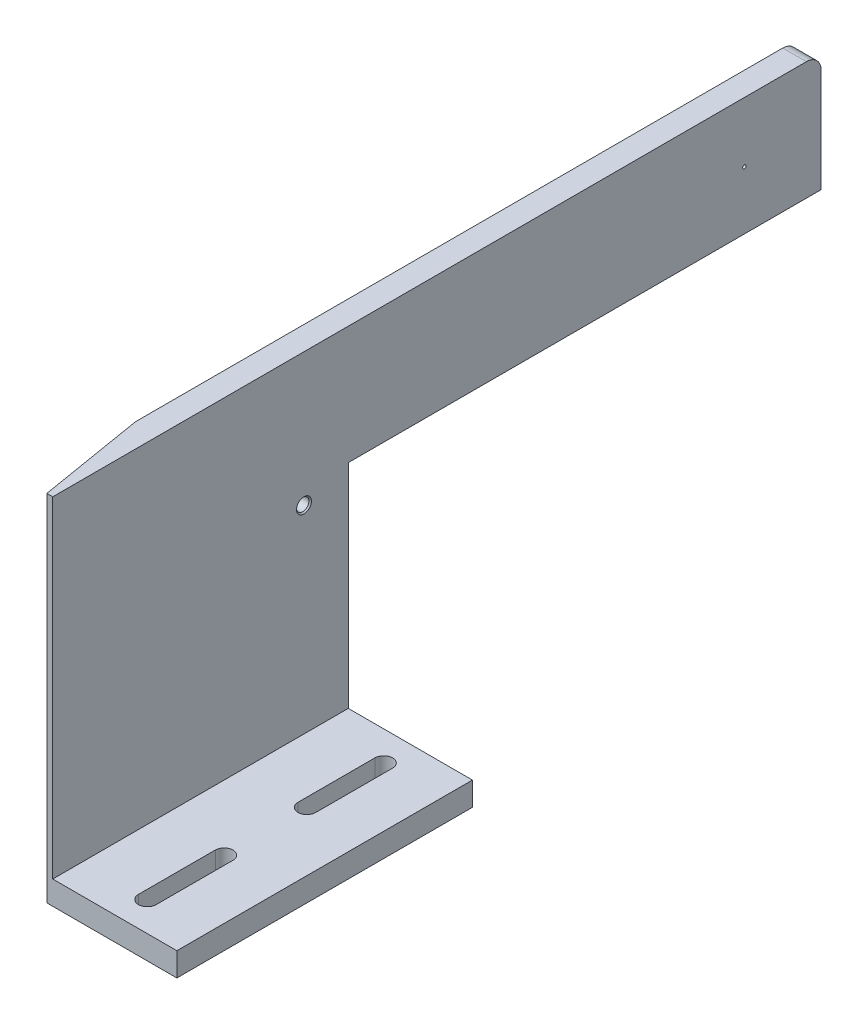
from build123d import *

# Parameters (mm, degrees)
BOSS_EXTRUDE1_DEPTH         = 260
SKETCH2_W                   = 160
SKETCH2_H                   = 80
CUT_EXTRUDE1_DEPTH          = 291.688837075
CUT_EXTRUDE2_DEPTH          = 220
CUT_EXTRUDE3_DEPTH          = 291.688837075
M5_TAPPED_HOLE1_D           = 4.2
M5_TAPPED_HOLE1_DEPTH       = 6
M5_TAPPED_HOLE1_CSINK_D     = 5.05
M5_TAPPED_HOLE1_CSINK_ANGLE = 90
M5_TAPPED_HOLE1_TIP         = 1.2618073
FILLET1_R                   = 5
SKETCH6_R                   = 0.6
CUT_EXTRUDE4_DEPTH          = 290.420109875


with BuildPart() as part:
    # Sketch1 → Boss-Extrude1 (new body)
    with BuildSketch(Plane.XY):
        Polygon((0, 0), (0, 120), (8, 120), (8, 8), (50, 8), (50, 0), align=None)
    extrude(amount=BOSS_EXTRUDE1_DEPTH)

    # Sketch2 → Cut-Extrude1 (cut, through all)
    with BuildSketch(Plane(origin=(50, 0, 0), x_dir=(0, 0, -1), z_dir=(1, 0, 0))):
        with Locations((-80, 40)):
            Rectangle(SKETCH2_W, SKETCH2_H)
    extrude(amount=-CUT_EXTRUDE1_DEPTH, mode=Mode.SUBTRACT)

    # Sketch3 → Cut-Extrude2 (cut)
    with BuildSketch(Plane(origin=(0, 8, 0), x_dir=(1, 0, 0), z_dir=(0, 1, 0))):
        with BuildLine():
            Line((27, -250), (27, -224))
            ThreePointArc((27, -224), (30, -221), (33, -224))
            Line((33, -224), (33, -250))
            ThreePointArc((33, -250), (30, -253), (27, -250))
        make_face()
        with BuildLine():
            Line((27, -196), (27, -170))
            ThreePointArc((27, -170), (30, -167), (33, -170))
            Line((33, -170), (33, -196))
            ThreePointArc((33, -196), (30, -199), (27, -196))
        make_face()
    extrude(amount=-CUT_EXTRUDE2_DEPTH, mode=Mode.SUBTRACT)

    # Sketch4 → Cut-Extrude3 (cut, through all)
    with BuildSketch(Plane(origin=(0, 120, 0), x_dir=(1, 0, 0), z_dir=(0, 1, 0))):
        Polygon((6, -260), (0, -224), (0, -260), align=None)
    extrude(amount=-CUT_EXTRUDE3_DEPTH, mode=Mode.SUBTRACT)

    # M5 Tapped Hole1
    with Locations(Plane(origin=(8, 75, 175), x_dir=(0, 0, 1), z_dir=(1, 0, 0))):
        with Locations((0, 0)):
            CounterSinkHole(M5_TAPPED_HOLE1_D / 2, M5_TAPPED_HOLE1_CSINK_D / 2, depth=M5_TAPPED_HOLE1_DEPTH, counter_sink_angle=M5_TAPPED_HOLE1_CSINK_ANGLE)
            with Locations((0, 0, -(M5_TAPPED_HOLE1_DEPTH + M5_TAPPED_HOLE1_TIP / 2))):  # 118° drill point
                Cone(0, M5_TAPPED_HOLE1_D / 2, M5_TAPPED_HOLE1_TIP, mode=Mode.SUBTRACT)

    # Fillet1
    fillet1_edges = [part.edges().sort_by_distance(p)[0] for p in [
        (4, 120, 0),
    ]]
    fillet(fillet1_edges, radius=FILLET1_R)

    # Sketch6 → Cut-Extrude4 (cut, through all)
    with BuildSketch(Plane(origin=(8, 0, 0), x_dir=(0, 0, -1), z_dir=(1, 0, 0))):
        with Locations((-26, 99.679986911)):
            Circle(SKETCH6_R)
    extrude(amount=-CUT_EXTRUDE4_DEPTH, mode=Mode.SUBTRACT)


solid = part.part
